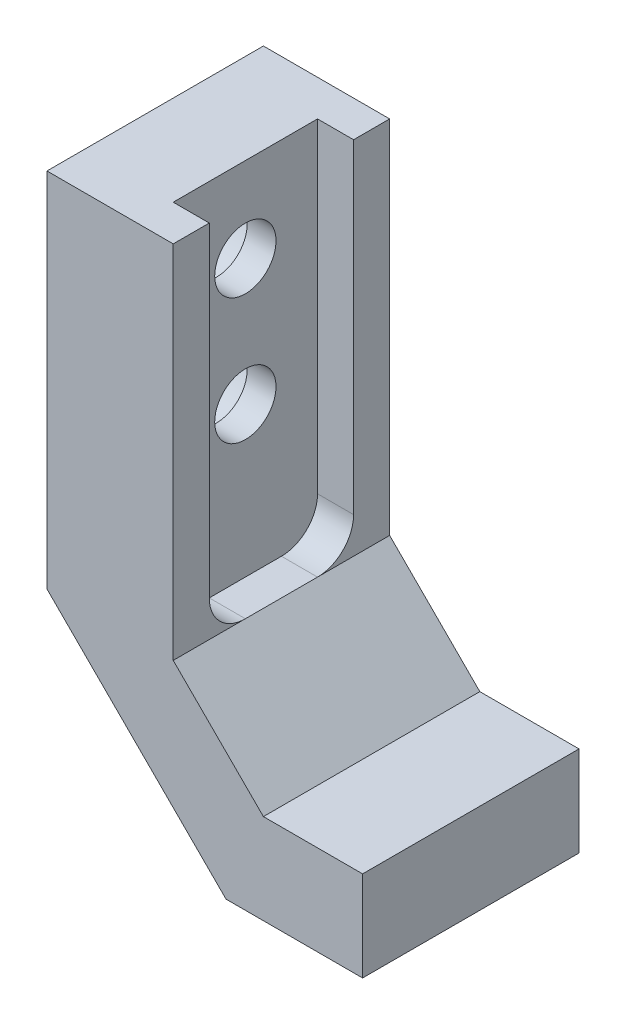
SolidWorks part; units mm, degrees
ref_plane "前视基准面" through (0, 0, 0) normal (0, 0, 1) x (1, 0, 0)
ref_plane "上视基准面" through (0, 0, 0) normal (0, 1, 0) x (1, 0, 0)
ref_plane "右视基准面" through (0, 0, 0) normal (1, 0, 0) x (0, 0, -1)
sketch "草图1" plane through (0, 0, 0) normal (0, 0, 1) x (1, 0, 0)
  line L0 (0, 0) -> (0, -20.0711)
  line L1 (0, -20.0711) -> (9.9289, -30)
  line L3 (12, -25) -> (7, -20)
  line L4 (7, -20) -> (7, 0)
  line L5 (7, 0) -> (0, 0)
  line L6 (12, -25) -> (17.5, -25)
  line L7 (17.5, -25) -> (17.5, -30)
  line L8 (17.5, -30) -> (9.9289, -30)
  dimension "D1" = 5
  dimension "D2" = 20
  dimension "D3" = 7
  dimension "D4" = 10.5
  dimension "D5" = 135
  dimension "D6" = 5
  dimension "D7" = 10
extrude "凸台-拉伸1" add sketch "草图1" along normal mid plane 12
sketch "草图2" plane through (0, 0, 0) normal (0, 1, 0) x (1, 0, 0)
  line L0 (7, -6) -> (7, 6) construction
  line L1 (7, 4) -> (5, 4)
  line L2 (7, 4) -> (7, -4)
  line L3 (7, -4) -> (5, -4)
  line L4 (5, 4) -> (5, -4)
  point P6 (5, 0)
  dimension "D1" = 8
  dimension "D2" = 2
extrude "切除-拉伸1" cut sketch "草图2" against normal blind 20
fillet "圆角1" radius 2 2 edges at (6, -20, 4) (6, -20, -4)
sketch "草图5" plane through (0, 0, 0) normal (-1, 0, 0) x (0, 0, 1)
  point P0 (0, -4.7)
  point P3 (0, -11.7)
hole_wizard "M3 六角圆柱头螺钉的柱形沉头孔1" positions "草图5" profile "草图4" counterbore size "M3" standard "GB" end condition through all
sketch "草图4" plane through (0, -4.7, 0) normal (0, 1, 0) x (0, 0, 1)
  line L0 (0, 0) -> (0, 17.5)
  line L1 (0, 17.5) -> (1.7, 17.5)
  line L3 (1.7, 17.5) -> (1.7, 3.4)
  line L4 (1.7, 3.4) -> (3, 3.4)
  line L5 (3, 3.4) -> (3, 0)
  line L7 (3, 0) -> (0, 0)
  line L11 (0, -6.35) -> (0, 107.95) construction
  dimension "通孔孔直径" = 3.4
  dimension "通孔孔深度" = 17.5
  dimension "柱形沉头孔直径" = 6
  dimension "柱形沉头孔深度" = 3.4
